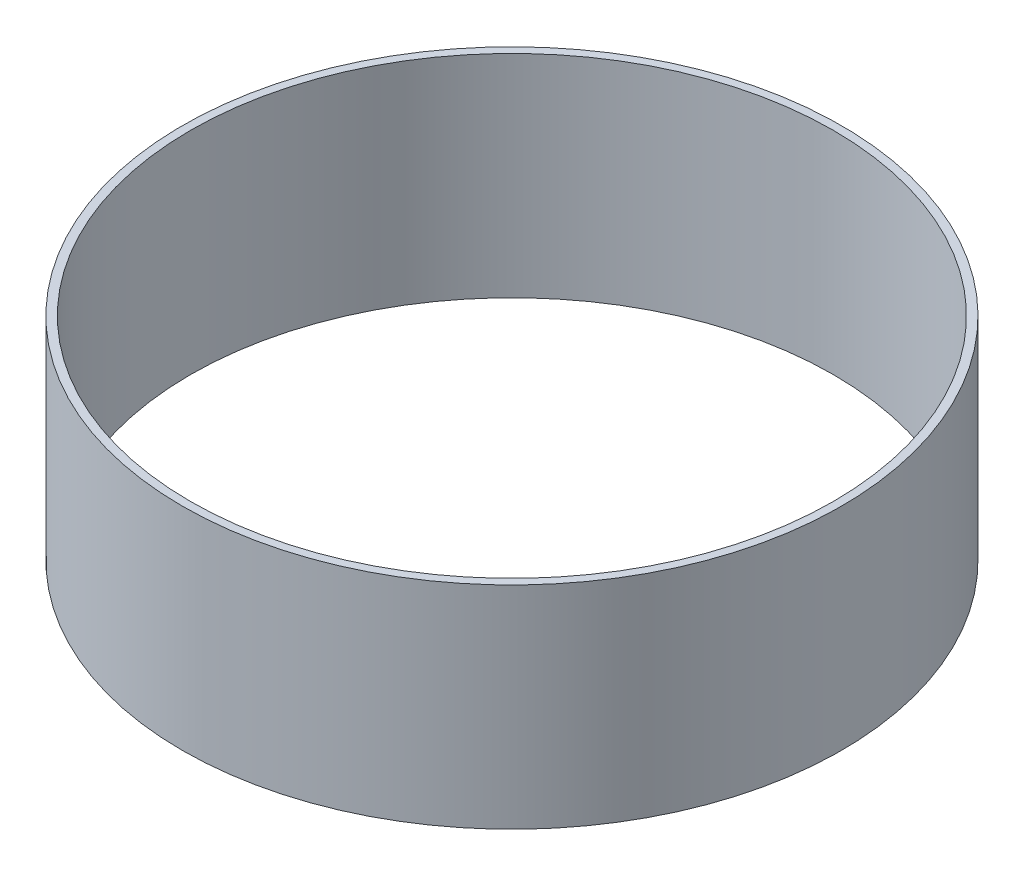
from build123d import *

# Parameters (mm, degrees)
SKETCH1_R           = 405
SKETCH1_R_2         = 395
BOSS_EXTRUDE1_DEPTH = 260


with BuildPart() as part:
    # Sketch1 → Boss-Extrude1 (new body)
    with BuildSketch(Plane(origin=(0, 0, 0), x_dir=(1, 0, 0), z_dir=(0, 1, 0))):
        with Locations(Location((0, 0, 0), (0, 0, 270))):
            Circle(SKETCH1_R)
        with Locations(Location((0, 0, 0), (0, 0, 270))):
            Circle(SKETCH1_R_2, mode=Mode.SUBTRACT)
    extrude(amount=BOSS_EXTRUDE1_DEPTH)


solid = part.part
